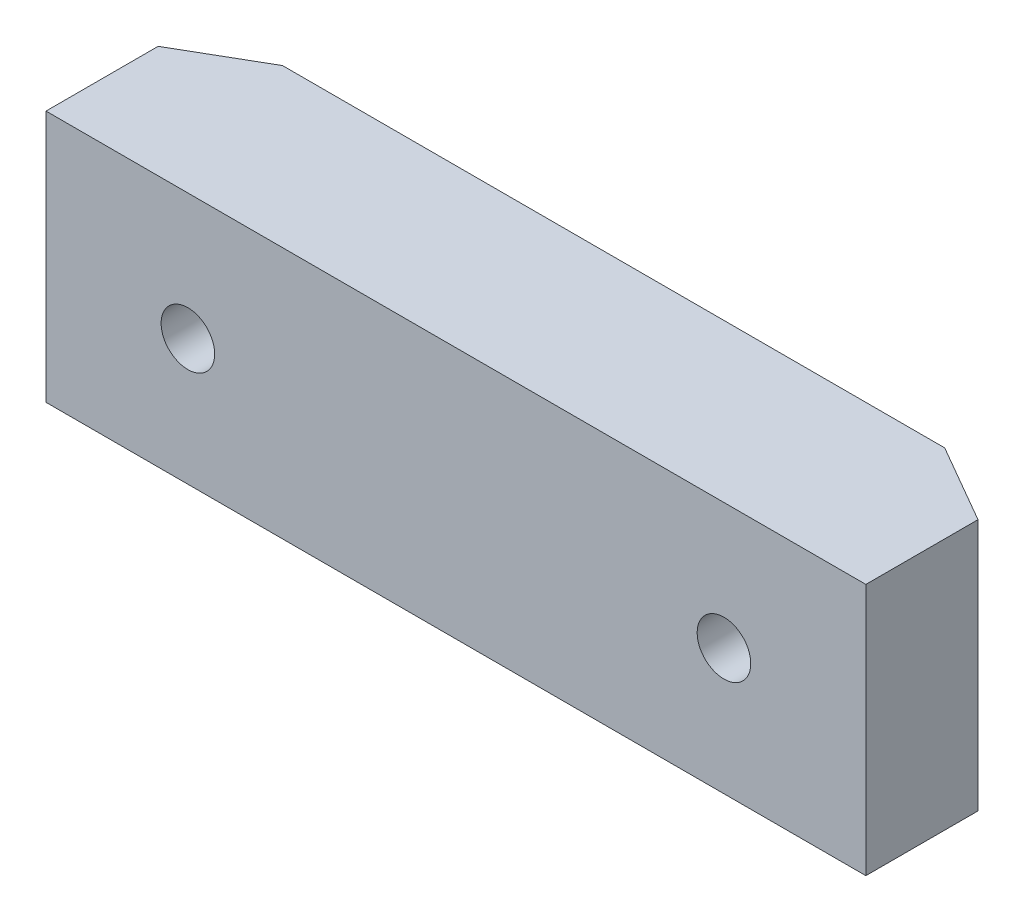
from build123d import *

# Parameters (mm, degrees)
SKETCH_1_W                = 52
SKETCH_1_H                = 16
EXTRUDE_1_DEPTH           = 10
HOLE_WIZARD_1_D           = 3.4
HOLE_WIZARD_1_DEPTH       = 38
HOLE_WIZARD_1_CBORE_D     = 6
HOLE_WIZARD_1_CBORE_DEPTH = 3.4
HOLE_WIZARD_1_TIP         = 1.021463052
CHAMFER_1_SIZE            = 5
CHAMFER_1_SIZE2           = 2.886751346
CHAMFER_2_SIZE            = 5
CHAMFER_2_SIZE2           = 2.886751346


with BuildPart() as part:
    # 草图1 → 凸台-拉伸1 (new body)
    with BuildSketch(Plane.XY):
        Rectangle(SKETCH_1_W, SKETCH_1_H)
    extrude(amount=EXTRUDE_1_DEPTH)

    # 打孔尺寸(%根据)内六角圆柱头螺钉的类型1
    with Locations(Plane(origin=(0, 0, 0), x_dir=(-1, 0, 0), z_dir=(0, 0, -1))):
        with Locations((-17, 0), (17, 0)):
            CounterBoreHole(HOLE_WIZARD_1_D / 2, HOLE_WIZARD_1_CBORE_D / 2, HOLE_WIZARD_1_CBORE_DEPTH, depth=HOLE_WIZARD_1_DEPTH)
            with Locations((0, 0, -(HOLE_WIZARD_1_DEPTH + HOLE_WIZARD_1_TIP / 2))):  # 118° drill point
                Cone(0, HOLE_WIZARD_1_D / 2, HOLE_WIZARD_1_TIP, mode=Mode.SUBTRACT)

    # 倒角1
    chamfer_1_edges = [part.edges().sort_by_distance(p)[0] for p in [
        (26, 0, 0),
    ]]
    chamfer_1_side = [part.faces().sort_by_distance(p)[0] for p in [
        (0, 0, 0),
    ]]
    chamfer(chamfer_1_edges, length=CHAMFER_1_SIZE, length2=CHAMFER_1_SIZE2, reference=chamfer_1_side[0])

    # 倒角2
    chamfer_2_edges = [part.edges().sort_by_distance(p)[0] for p in [
        (-26, 0, 0),
    ]]
    chamfer_2_side = [part.faces().sort_by_distance(p)[0] for p in [
        (-2.703280464, 0, 0),
    ]]
    chamfer(chamfer_2_edges, length=CHAMFER_2_SIZE, length2=CHAMFER_2_SIZE2, reference=chamfer_2_side[0])


solid = part.part
